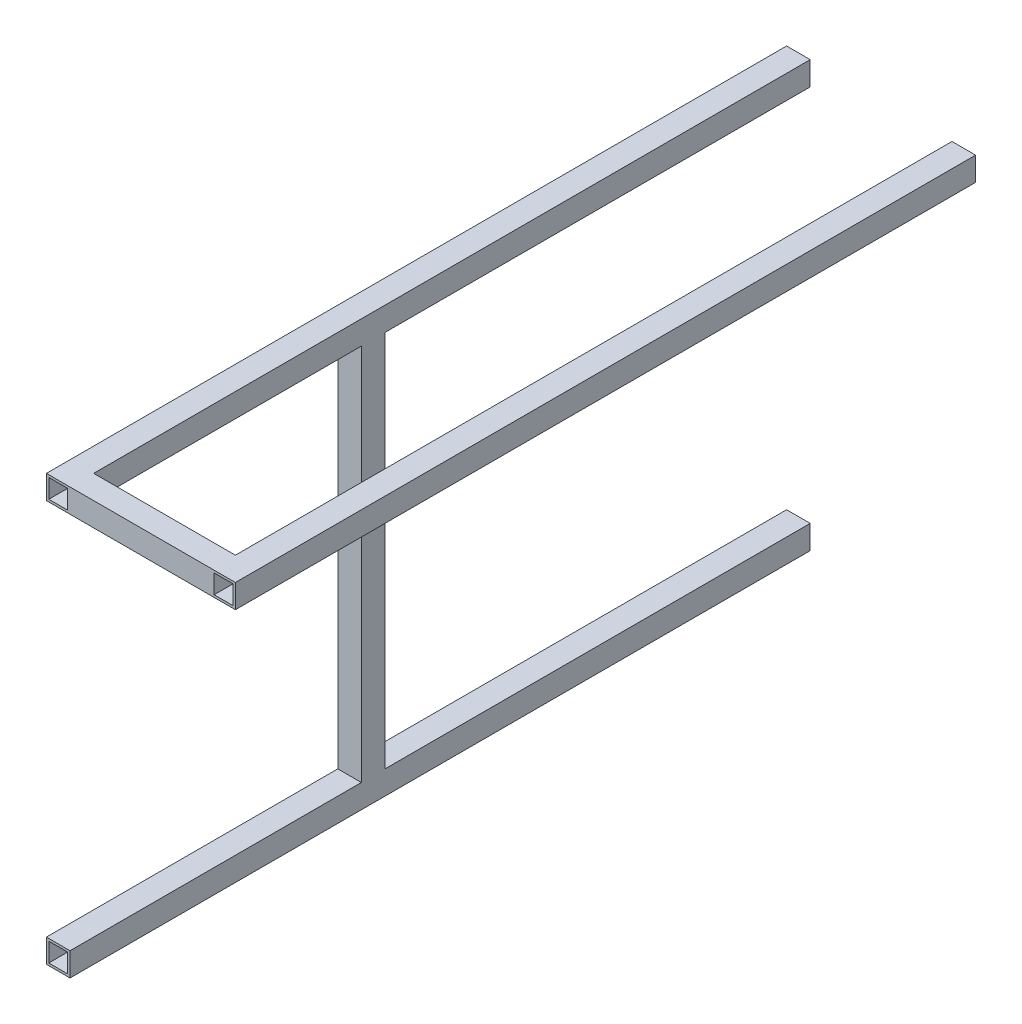
from build123d import *

# Parameters (mm, degrees)
SKETCH_1_W          = 30
SKETCH_1_H          = 30
SKETCH_1_W_2        = 24
SKETCH_1_H_2        = 24
EXTRUDE_1_DEPTH     = 940
EXTRUDE_1_2_DEPTH   = 940
EXTRUDE_1_3_DEPTH   = 940
SKETCH_3_W          = 30
SKETCH_3_H          = 30
SKETCH_3_W_2        = 24
SKETCH_3_H_2        = 24
EXTRUDE_2_DEPTH     = 480
SKETCH_4_W          = 30
SKETCH_4_H          = 480
CUT_EXTRUDE_1_DEPTH = 37
SKETCH_5_W          = 30
SKETCH_5_H          = 480
EXTRUDE_3_DEPTH     = 30
SKETCH_6_W          = 30
SKETCH_6_H          = 30
EXTRUDE_4_DEPTH     = 180


with BuildPart() as part:
    # 草图1 → 凸台-拉伸1 (new body)
    with BuildSketch(Plane.XY):
        with Locations((15, 15)):
            Rectangle(SKETCH_1_W, SKETCH_1_H)
        with Locations((15, 15)):
            Rectangle(SKETCH_1_W_2, SKETCH_1_H_2, mode=Mode.SUBTRACT)
    extrude(amount=EXTRUDE_1_DEPTH)



with BuildPart() as body_2:
    # 草图1 → Extrude 1 2 (new body)
    with BuildSketch(Plane.XY):
        with Locations((225, 15)):
            Rectangle(SKETCH_1_W, SKETCH_1_H)
        with Locations((225, 15)):
            Rectangle(SKETCH_1_W_2, SKETCH_1_H_2, mode=Mode.SUBTRACT)
    extrude(amount=EXTRUDE_1_2_DEPTH)



with BuildPart() as body_3:
    # 草图1 → Extrude 1 3 (new body)
    with BuildSketch(Plane.XY):
        with Locations((15, -495)):
            Rectangle(SKETCH_1_W, SKETCH_1_H)
        with Locations((15, -495)):
            Rectangle(SKETCH_1_W_2, SKETCH_1_H_2, mode=Mode.SUBTRACT)
    extrude(amount=EXTRUDE_1_3_DEPTH)


with BuildPart() as part_1:
    add(part.part)

    add(body_3.part)  # 凸台-拉伸2 merges body 3
    # 草图3 → 凸台-拉伸2 (add)
    with BuildSketch(Plane.XZ):
        with Locations((15, 385)):
            Rectangle(SKETCH_3_W, SKETCH_3_H)
        with Locations((15, 385)):
            Rectangle(SKETCH_3_W_2, SKETCH_3_H_2, mode=Mode.SUBTRACT)
    extrude(amount=EXTRUDE_2_DEPTH)

    # 草图4 → 切除-拉伸1 (cut)
    with BuildSketch(Plane.ZY):
        with Locations((385, -240)):
            Rectangle(SKETCH_4_W, SKETCH_4_H)
    extrude(amount=-CUT_EXTRUDE_1_DEPTH, mode=Mode.SUBTRACT)


with BuildPart() as cut_extrude_1_piece_1:
    # of the separate pieces the step leaves, piece 1, a body of its own (cut_extrude_1_pieces)
    add(part_1.part.solids().sort_by_distance((0, 0, 940))[0])



with BuildPart() as cut_extrude_1_piece_2:
    # of the separate pieces the step leaves, piece 2, a body of its own (cut_extrude_1_pieces)
    add(part_1.part.solids().sort_by_distance((0, -510, 0))[0])


with BuildPart() as cut_extrude_1_piece_1_1:
    add(cut_extrude_1_piece_1.part)

    add(cut_extrude_1_piece_2.part)  # 凸台-拉伸3 merges 切除-拉伸1 piece 2
    # 草图5 → 凸台-拉伸3 (add)
    with BuildSketch(Plane.ZY):
        with Locations((555, -240)):
            Rectangle(SKETCH_5_W, SKETCH_5_H)
    extrude(amount=-EXTRUDE_3_DEPTH)


with BuildPart() as body_2_1:
    add(body_2.part)

    add(cut_extrude_1_piece_1_1.part)  # 凸台-拉伸4 merges 切除-拉伸1 piece 1
    # 草图6 → 凸台-拉伸4 (add)
    with BuildSketch(Plane.ZY.offset(-210)):
        with Locations((925, 15)):
            Rectangle(SKETCH_6_W, SKETCH_6_H)
    extrude(amount=EXTRUDE_4_DEPTH)


solid = body_2_1.part
